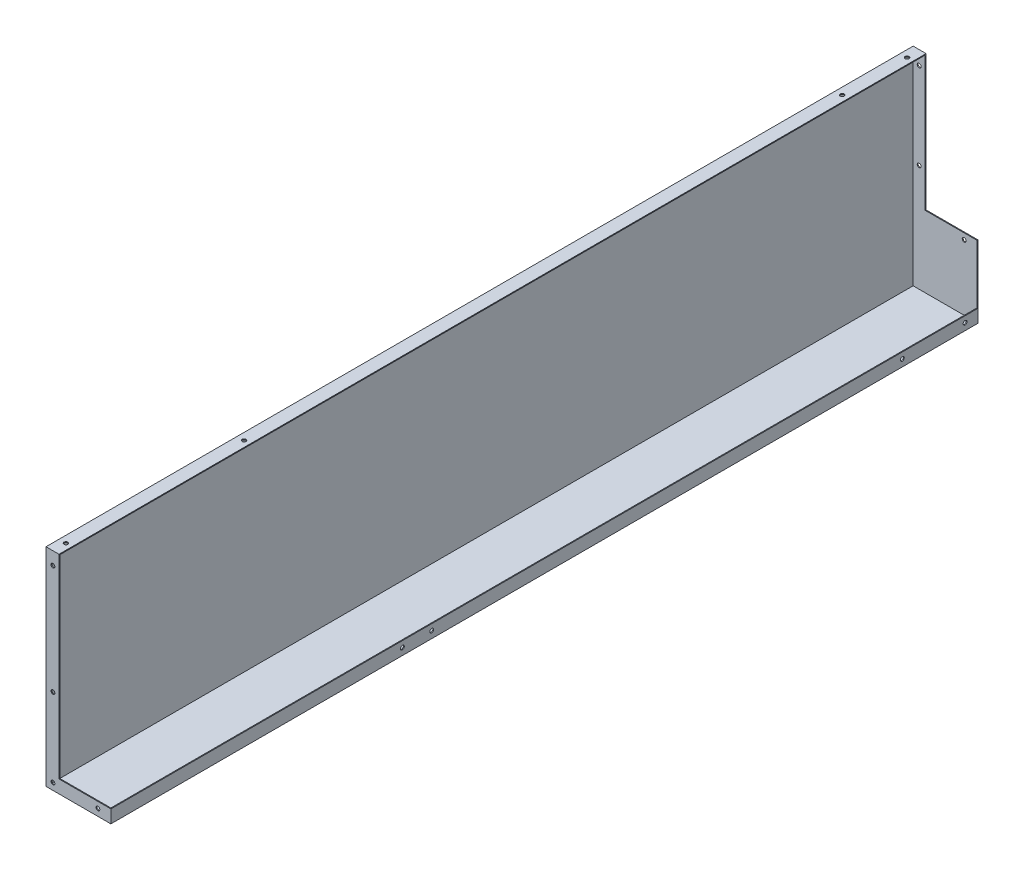
SolidWorks part; units mm, degrees
ref_plane "前视基准面" through (0, 0, 0) normal (0, 0, 1) x (1, 0, 0)
ref_plane "上视基准面" through (0, 0, 0) normal (0, 1, 0) x (1, 0, 0)
ref_plane "右视基准面" through (0, 0, 0) normal (1, 0, 0) x (0, 0, -1)
sketch "草图1" plane through (0, 0, 0) normal (0, 0, 1) x (1, 0, 0)
  line L0 (0, 480) -> (0, 0)
  line L1 (0, 0) -> (150, 0)
  dimension "D1" = 480
  dimension "D2" = 150
extrude "拉伸-薄壁1" add sketch "草图1" along normal blind 2005 thin thin type one direction reverse wall 2
sketch "草图3" plane through (2, 0, 0) normal (1, 0, 0) x (0, 0, -1)
  line L7 (-2003, 2) -> (-2003, 478)
  line L8 (-2003, 478) -> (-2, 478)
  line L9 (-2, 478) -> (-2, 2)
  line L10 (0, 480) -> (0, 2)
  line L11 (-2005, 480) -> (0, 480)
  line L12 (-2005, 2) -> (-2005, 480)
  line L13 (0, 480) -> (0, 2)
  line L14 (-2005, 480) -> (0, 480)
  line L15 (-2005, 2) -> (-2005, 480)
  line L16 (-2005, 2) -> (-2003, 2)
  line L17 (-2, 2) -> (0, 2)
  dimension "D1" = 0
  dimension "D2" = 2
extrude "凸台-拉伸1" add sketch "草图3" along normal blind 28
sketch "草图4" plane through (0, 2, 0) normal (0, 1, 0) x (1, 0, 0)
  line L0 (148, -2003) -> (148, 0)
  line L1 (30, 0) -> (150, 0) construction
  line L2 (148, 0) -> (150, 0)
  line L6 (30, -2003) -> (148, -2003)
  line L9 (30, -2005) -> (150, -2005)
  line L10 (150, -2005) -> (150, 0)
  line L11 (150, 0) -> (30, 0)
  line L12 (30, -2005) -> (150, -2005)
  line L13 (150, -2005) -> (150, 0)
  line L15 (30, -2003) -> (30, -2005)
  line L17 (150, 0) -> (30, 0) construction
  line L18 (148, -2) -> (30, -2) construction
  line L19 (148, -2003) -> (148, -2) construction
  dimension "D1" = 0
  dimension "D2" = 2
extrude "凸台-拉伸2" add sketch "草图4" along normal blind 28
sketch "草图5" plane through (0, 2, 0) normal (0, 1, 0) x (1, 0, 0)
  line L0 (30, 0) -> (30, -2005) construction
  line L1 (150, 0) -> (30, 0)
  line L2 (150, 0) -> (150, -2)
  line L3 (150, -2) -> (30, -2)
  line L4 (30, 0) -> (30, -2)
  dimension "D1" = 2
extrude "凸台-拉伸3" add sketch "草图5" along normal blind 165
sketch "草图7" plane through (0, 0, 2) normal (0, 0, 1) x (1, 0, 0)
  line L0 (16, 478) -> (16, -60.8022) construction
  line L1 (30, 478) -> (2, 478) construction
  line L2 (150, 153) -> (-197.568, 153) construction
  line L3 (150, 167) -> (150, 30) construction
  line L4 (30, 167) -> (150, 167) construction
  line L5 (0, 480) -> (30, 480) construction
  circle A0 centre (120, 153) radius 4.5
  circle A1 centre (16, 450) radius 4.5
  circle A2 centre (16, 250) radius 4.5
  dimension "D2" = 9
  dimension "D3" = 9
  dimension "D4" = 9
  dimension "D5" = 30
  dimension "D6" = 30
  dimension "D7" = 200
  dimension "D1" = 14
extrude "切除-拉伸2" cut sketch "草图7" against normal blind 10
sketch "草图8" plane through (0, 478, 0) normal (0, -1, 0) x (1, 0, 0)
  line L0 (16, 2) -> (16, 209.1635) construction
  line L1 (30, 2) -> (2, 2) construction
  line L2 (0, 0) -> (30, 0) construction
  circle A0 centre (16, 30) radius 4.5
  circle A1 centre (16, 180) radius 4.5
  dimension "D1" = 9
  dimension "D2" = 9
  dimension "D3" = 150
  dimension "D4" = 30
extrude "切除-拉伸3" cut sketch "草图8" against normal blind 76
sketch "草图9" plane through (0, 478, 0) normal (0, -1, 0) x (1, 0, 0)
  line L0 (16, 2003) -> (16, 1584.8247) construction
  line L1 (30, 2003) -> (2, 2003) construction
  line L2 (0, 2005) -> (30, 2005) construction
  circle A0 centre (16, 1975) radius 4.5
  circle A1 centre (16, 1563) radius 4.5
  dimension "D1" = 9
  dimension "D2" = 9
  dimension "D3" = 30
  dimension "D4" = 412
extrude "切除-拉伸4" cut sketch "草图9" against normal blind 10
sketch "草图10" plane through (0, 0, 2005) normal (0, 0, 1) x (1, 0, 0)
  line L0 (16, 504.8239) -> (16, 255.5129) construction
  line L1 (30, 480) -> (30, 30) construction
  line L2 (0, 480) -> (30, 480) construction
  line L7 (150, 30) -> (150, 0) construction
  line L9 (16, 16) -> (150, 16)
  line L10 (16, 480) -> (16, 16)
  line L11 (16, 16) -> (150, 16) construction
  line L12 (16, 480) -> (16, 16) construction
  circle A0 centre (16, 450) radius 4.5
  circle A1 centre (16, 197) radius 4.5
  circle A2 centre (16, 16) radius 4.5
  circle A3 centre (120, 16) radius 4.5
  dimension "D2" = 9
  dimension "D3" = 30
  dimension "D4" = 9
  dimension "D5" = 253
  dimension "D7" = 9
  dimension "D8" = 9
  dimension "D9" = 30
  dimension "D1" = 14
  dimension "D6" = 14
extrude "切除-拉伸5" cut sketch "草图10" against normal blind 10
sketch "草图11" plane through (150, 0, 0) normal (1, 0, 0) x (0, 0, -1)
  line L6 (-2005, 16) -> (-2, 16)
  line L7 (-2005, 16) -> (-2, 16) construction
  line L8 (0, 167) -> (0, 0) construction
  circle A0 centre (-30, 16) radius 4.5
  circle A1 centre (-175, 16) radius 4.5
  circle A2 centre (-1331, 16) radius 4.5
  circle A3 centre (-1263, 16) radius 4.5
  dimension "D2" = 9
  dimension "D3" = 9
  dimension "D4" = 30
  dimension "D5" = 145
  dimension "D6" = 9
  dimension "D7" = 9
  dimension "D8" = 1263
  dimension "D9" = 68
  dimension "D1" = 14
extrude "切除-拉伸6" cut sketch "草图11" against normal blind 16
